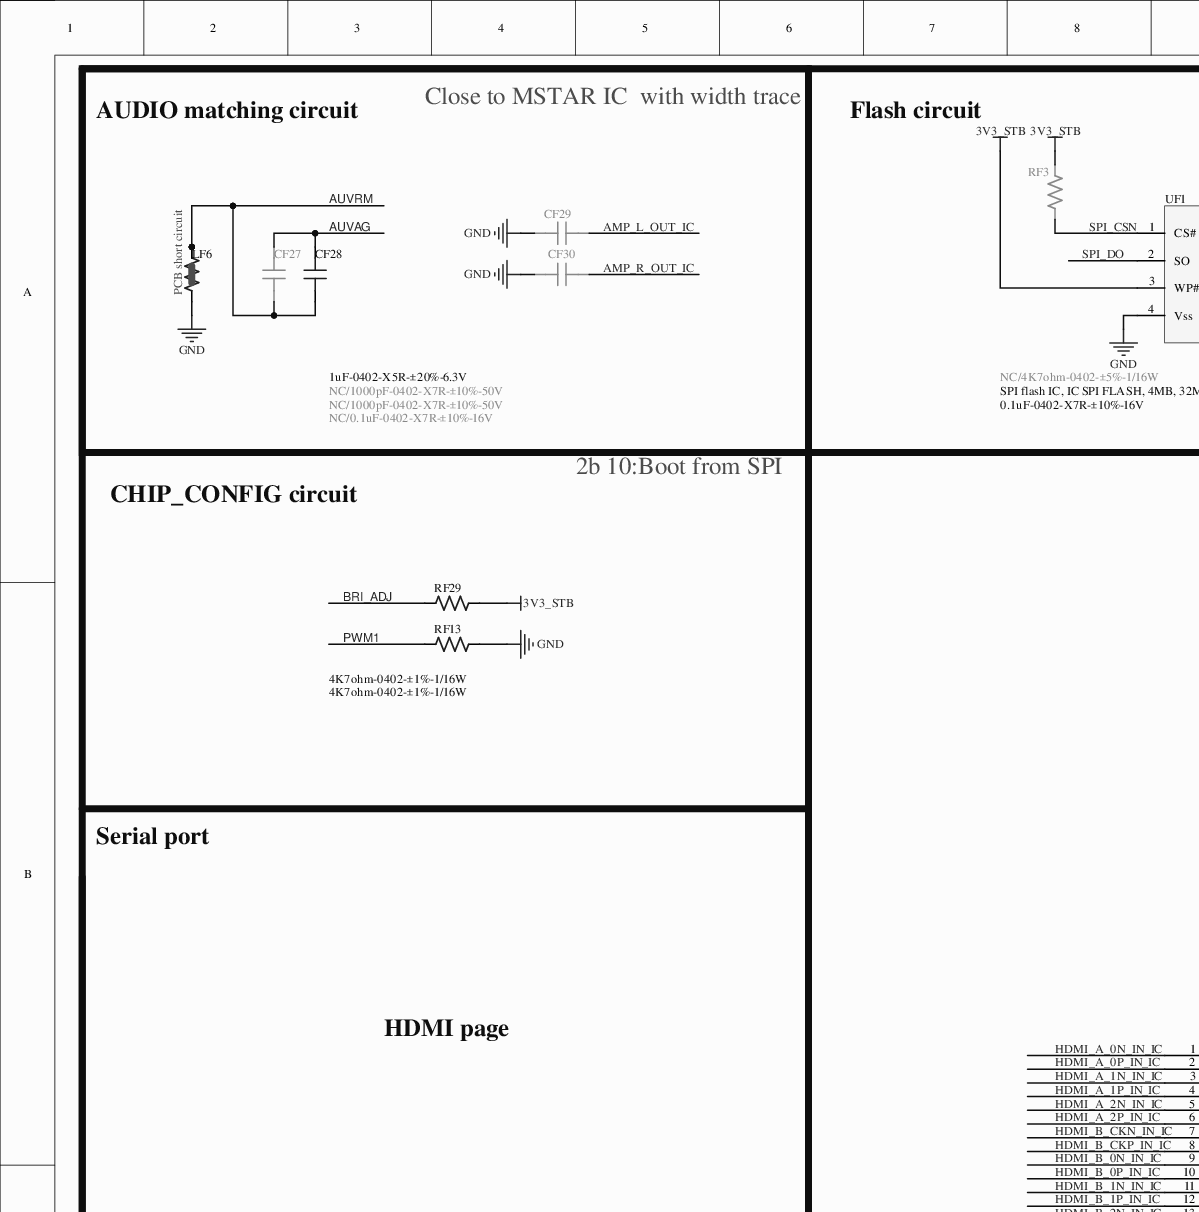
[diagram p0: MISC105950-36.SchDoc, top left]
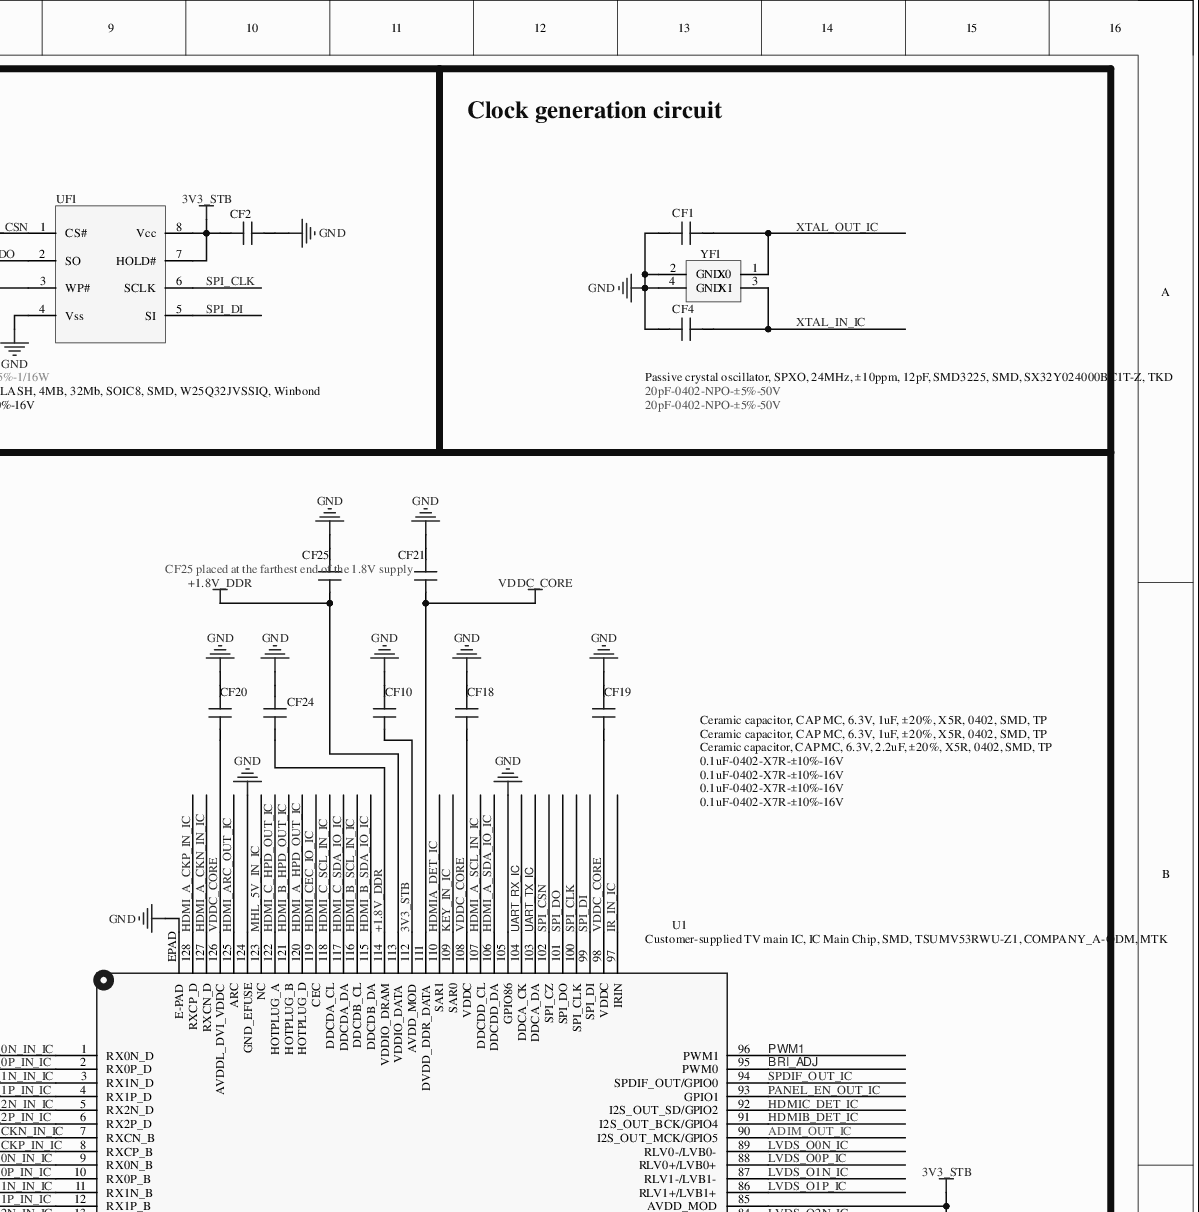
[diagram p1: MISC105950-36.SchDoc, top right]
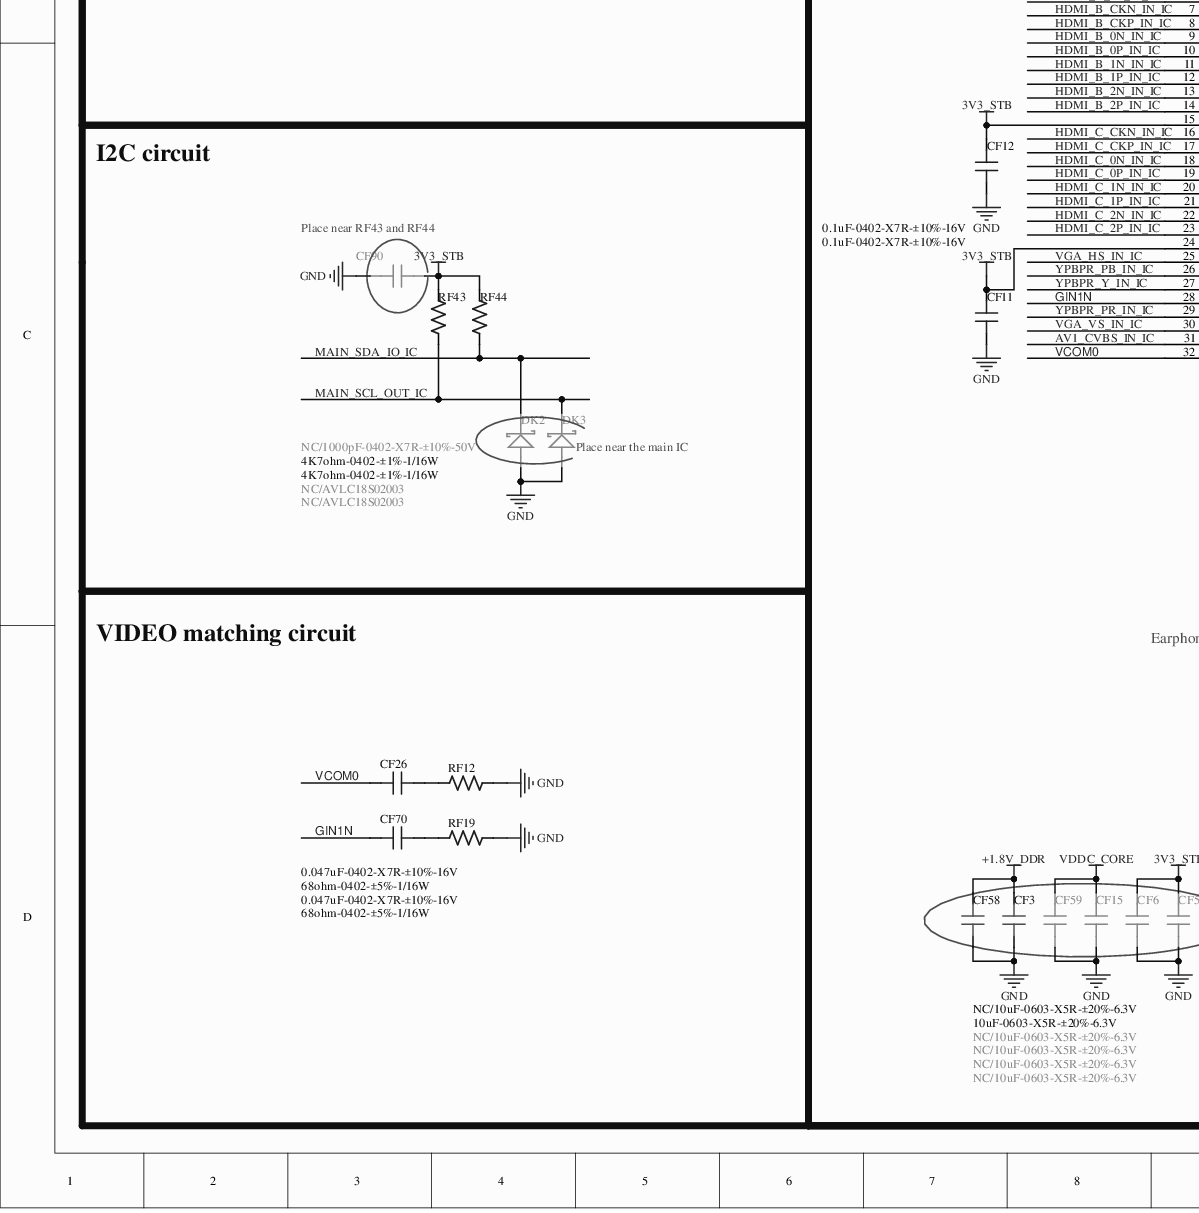
[diagram p2: MISC105950-36.SchDoc, bottom left]
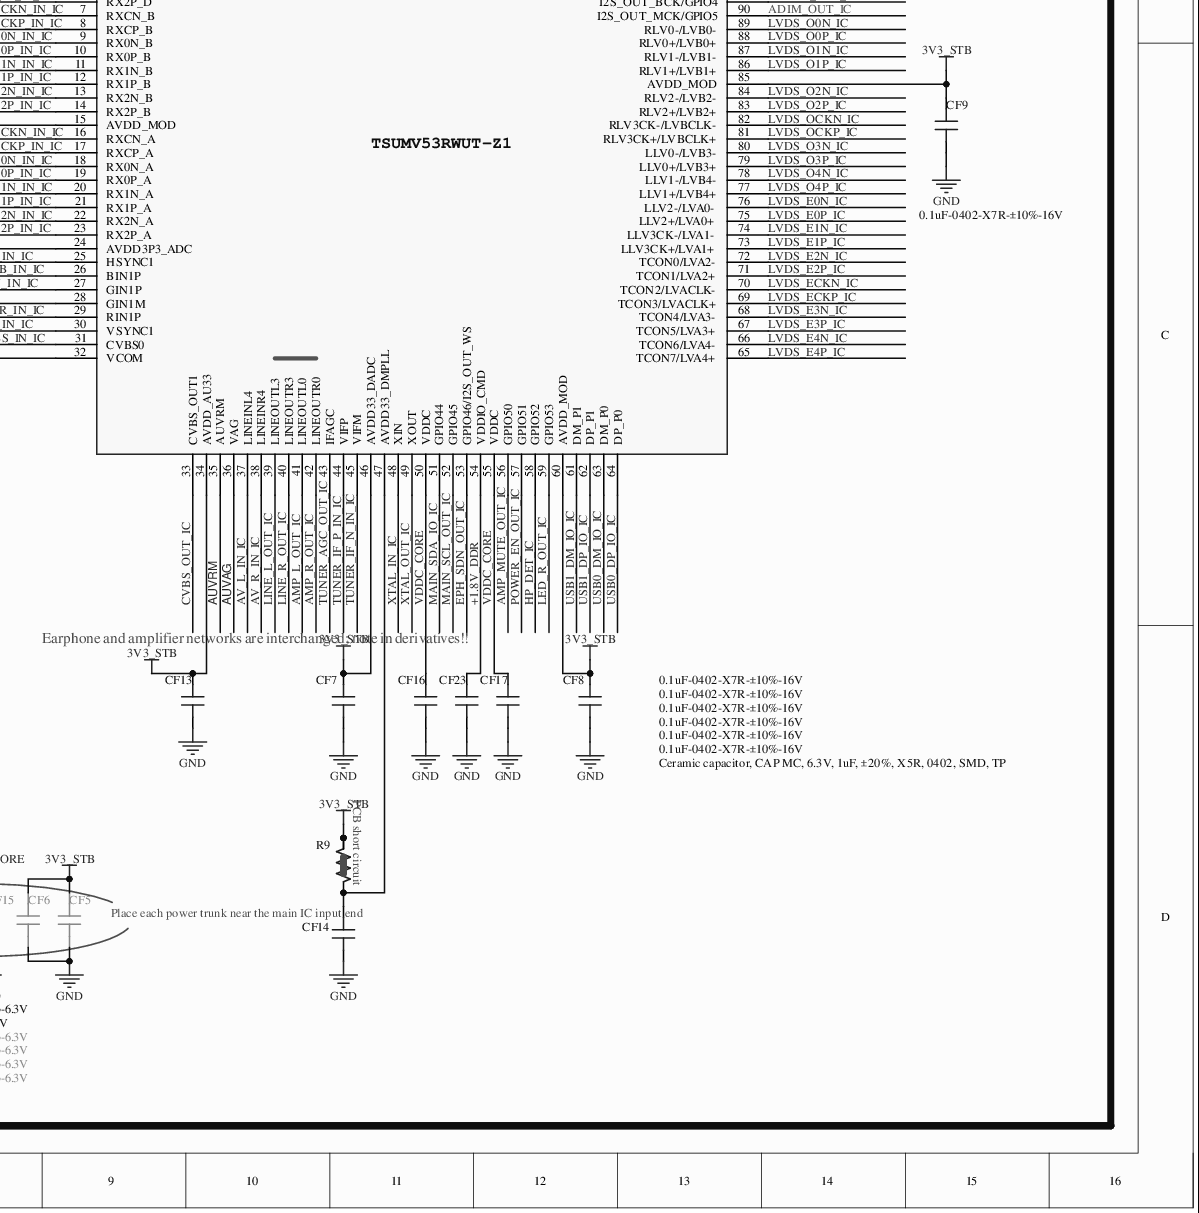
[diagram p3: MISC105950-36.SchDoc, bottom right]
# Altium project MISC105950-48.PrjPCB (part 4 of 8)

## Sheet MISC105950-36.SchDoc
size 426 x 431 mm

### Parts
CF1  20pF-0402-NPO-±5%-50V  [C0402]
CF2  0.1uF-0402-X7R-±10%-16V  [C0402]
CF3  10uF-0603-X5R-±20%-6.3V  [C0603]
CF4  20pF-0402-NPO-±5%-50V  [C0402]
CF5  NC/10uF-0603-X5R-±20%-6.3V  [C0603]
CF6  NC/10uF-0603-X5R-±20%-6.3V  [C0603]
CF7  0.1uF-0402-X7R-±10%-16V  [C0402]
CF8  0.1uF-0402-X7R-±10%-16V  [C0402]
CF9  0.1uF-0402-X7R-±10%-16V  [C0402]
CF10  0.1uF-0402-X7R-±10%-16V  [C0402]
CF11  0.1uF-0402-X7R-±10%-16V  [C0402]
CF12  0.1uF-0402-X7R-±10%-16V  [C0402]
CF13  0.1uF-0402-X7R-±10%-16V  [C0402]
CF14  0.1uF-0402-X7R-±10%-16V  [C0402]
CF15  NC/10uF-0603-X5R-±20%-6.3V  [C0603]
CF16  0.1uF-0402-X7R-±10%-16V  [C0402]
CF17  0.1uF-0402-X7R-±10%-16V  [C0402]
CF18  0.1uF-0402-X7R-±10%-16V  [C0402]
CF19  0.1uF-0402-X7R-±10%-16V  [C0402]
CF20  0.1uF-0402-X7R-±10%-16V  [C0402]
CF21  Ceramic capacitor, CAP MC, 6.3V, 1uF, ±20%, X5R, 0402, SMD, TP  [C0402]
CF23  Ceramic capacitor, CAP MC, 6.3V, 1uF, ±20%, X5R, 0402, SMD, TP  [C0402]
CF24  Ceramic capacitor, CAP MC, 6.3V, 1uF, ±20%, X5R, 0402, SMD, TP  [C0402]
CF25  Ceramic capacitor, CAP MC, 6.3V, 2.2uF, ±20%, X5R, 0402, SMD, TP  [C0402]
CF26  0.047uF-0402-X7R-±10%-16V  [C0402]
CF27  NC/0.1uF-0402-X7R-±10%-16V  [C0402]
CF28  1uF-0402-X5R-±20%-6.3V  [C0402]
CF29  NC/1000pF-0402-X7R-±10%-50V  [C0402]
CF30  NC/1000pF-0402-X7R-±10%-50V  [C0402]
CF58  NC/10uF-0603-X5R-±20%-6.3V  [C0603]
CF59  NC/10uF-0603-X5R-±20%-6.3V  [C0603]
CF70  0.047uF-0402-X7R-±10%-16V  [C0402]
CF90  NC/1000pF-0402-X7R-±10%-50V  [C0402]
DK2  NC/AVLC18S02003  [DIODE-S0402]
DK3  NC/AVLC18S02003  [DIODE-S0402]
LF6  NC/0ohm-0402-PCB  [R0402SC]  (value not drawn)
R9  NC/0ohm-0402-PCB  [R0402SC]  (value not drawn)
RF3  NC/4K7ohm-0402-±5%-1/16W  [R0402]
RF12  68ohm-0402-±5%-1/16W  [R0402]
RF13  4K7ohm-0402-±1%-1/16W  [R0402]
RF19  68ohm-0402-±5%-1/16W  [R0402]
RF29  4K7ohm-0402-±1%-1/16W  [R0402]
RF43  4K7ohm-0402-±1%-1/16W  [R0402]
RF44  4K7ohm-0402-±1%-1/16W  [R0402]
U1  Customer-supplied TV main IC, IC Main Chip, SMD, TSUMV53RWU-Z1, COMPANY_A-ODM, MTK  [QFN128/0.35-1]
UF1  SPI flash IC, IC SPI FLASH, 4MB, 32Mb, SOIC8, SMD, W25Q32JVSSIQ, Winbond  [SOIC8]
YF1  Passive crystal oscillator, SPXO, 24MHz, ±10ppm, 12pF, SMD3225, SMD, SX32Y024000BC1T-Z, TKD  [XTAL-S-3]

### Blocks framed on the sheet
Flash circuit: CF2 RF3 UF1
VIDEO matching circuit: CF26 CF70 RF12 RF19

### Nets
3V3_STB: CF2.2 CF5.2 CF6.2 CF7.2 CF8.2 CF9.2 CF10.2 CF11.1 CF12.2 CF13.2 CF90.1 R9.2 R9.3 RF3.2 RF29.2 RF43.1 RF44.1 U1.15(AVDD_MOD) U1.24(AVDD3P3_ADC) U1.34(AVDD_AU33) U1.46(AVDD33_DADC) U1.60(AVDD_MOD) U1.85(AVDD_MOD) U1.112(AVDD_MOD) UF1.3(WP#) UF1.7(HOLD#) UF1.8(Vcc)
+1.8V_DDR: CF3.2 CF23.2 CF24.2 CF25.1 CF58.2 U1.54(VDDIO_CMD) U1.113(VDDIO_DATA) U1.114(VDDIO_DRAM)
GND: CF1.1 CF2.1 CF3.1 CF4.1 CF5.1 CF6.1 CF7.1 CF8.1 CF9.1 CF10.1 CF11.2 CF12.1 CF13.1 CF14.1 CF15.1 CF16.1 CF17.1 CF18.2 CF19.2 CF20.1 CF21.2 CF23.1 CF24.1 CF25.2 CF29.2 CF30.2 CF58.1 CF59.1 CF90.2 DK2.A DK3.A LF6.1 RF12.2 RF13.2 RF19.2 U1.105(GPIO86) U1.124(GND_EFUSE) U1.EPAD(E-PAD) UF1.4(Vss) YF1.2(GND) YF1.4(GND)
VDDC_CORE: CF15.2 CF16.2 CF17.2 CF18.1 CF19.1 CF20.2 CF21.1 CF59.2 U1.50(VDDC) U1.55(VDDC) U1.98(VDDC) U1.108(VDDC) U1.111(DVDD_DDR_DATA) U1.126(AVDDL_DVI_VDDC)
ADIM_OUT_IC: U1.90(I2S_OUT_MCK/GPIO5)
AMP_L_OUT_IC: CF29.1 U1.41(LINEOUTL0)
AMP_MUTE_OUT_IC: U1.56(GPIO50)
AMP_R_OUT_IC: CF30.1 U1.42(LINEOUTR0)
AUVAG: CF27.2 CF28.2 U1.36(VAG)
AUVRM: CF27.1 CF28.1 LF6.2 LF6.3 U1.35(AUVRM)
AV1_CVBS_IN_IC: U1.31(CVBS0)
AV_L_IN_IC: U1.37(LINEINL4)
AV_R_IN_IC: U1.38(LINEINR4)
BRI_ADJ: RF29.1 U1.95(PWM0)
CVBS_OUT_IC: U1.33(CVBS_OUT1)
EPH_SDN_OUT_IC: U1.53(GPIO46/I2S_OUT_WS)
GIN1N: CF70.1 U1.28(GIN1M)
HDMI_A_0N_IN_IC: U1.1(RX0N_D)
HDMI_A_0P_IN_IC: U1.2(RX0P_D)
HDMI_A_1N_IN_IC: U1.3(RX1N_D)
HDMI_A_1P_IN_IC: U1.4(RX1P_D)
HDMI_A_2N_IN_IC: U1.5(RX2N_D)
HDMI_A_2P_IN_IC: U1.6(RX2P_D)
HDMI_A_CKN_IN_IC: U1.127(RXCN_D)
HDMI_A_CKP_IN_IC: U1.128(RXCP_D)
HDMI_A_HPD_OUT_IC: U1.120(HOTPLUG_D)
HDMI_A_SCL_IN_IC: U1.107(DDCDD_CL)
HDMI_A_SDA_IO_IC: U1.106(DDCDD_DA)
HDMI_ARC_OUT_IC: U1.125(ARC)
HDMI_B_0N_IN_IC: U1.9(RX0N_B)
HDMI_B_0P_IN_IC: U1.10(RX0P_B)
HDMI_B_1N_IN_IC: U1.11(RX1N_B)
HDMI_B_1P_IN_IC: U1.12(RX1P_B)
HDMI_B_2N_IN_IC: U1.13(RX2N_B)
HDMI_B_2P_IN_IC: U1.14(RX2P_B)
HDMI_B_CKN_IN_IC: U1.7(RXCN_B)
HDMI_B_CKP_IN_IC: U1.8(RXCP_B)
HDMI_B_HPD_OUT_IC: U1.121(HOTPLUG_B)
HDMI_B_SCL_IN_IC: U1.116(DDCDB_CL)
HDMI_B_SDA_IO_IC: U1.115(DDCDB_DA)
HDMI_C_0N_IN_IC: U1.18(RX0N_A)
HDMI_C_0P_IN_IC: U1.19(RX0P_A)
HDMI_C_1N_IN_IC: U1.20(RX1N_A)
HDMI_C_1P_IN_IC: U1.21(RX1P_A)
HDMI_C_2N_IN_IC: U1.22(RX2N_A)
HDMI_C_2P_IN_IC: U1.23(RX2P_A)
HDMI_C_CKN_IN_IC: U1.16(RXCN_A)
HDMI_C_CKP_IN_IC: U1.17(RXCP_A)
HDMI_C_HPD_OUT_IC: U1.122(HOTPLUG_A)
HDMI_C_SCL_IN_IC: U1.118(DDCDA_CL)
HDMI_C_SDA_IO_IC: U1.117(DDCDA_DA)
HDMI_CEC_IO_IC: U1.119(CEC)
HDMIA_DET_IC: U1.110(SAR1)
HDMIB_DET_IC: U1.91(I2S_OUT_BCK/GPIO4)
HDMIC_DET_IC: U1.92(I2S_OUT_SD/GPIO2)
HP_DET_IC: U1.58(GPIO52)
IR_IN_IC: U1.97(IRIN)
KEY_IN_IC: U1.109(SAR0)
LED_R_OUT_IC: U1.59(GPIO53)
LINE_L_OUT_IC: U1.39(LINEOUTL3)
LINE_R_OUT_IC: U1.40(LINEOUTR3)
LVDS_E0N_IC: U1.76(LLV2-/LVA0-)
LVDS_E0P_IC: U1.75(LLV2+/LVA0+)
LVDS_E1N_IC: U1.74(LLV3CK-/LVA1-)
LVDS_E1P_IC: U1.73(LLV3CK+/LVA1+)
LVDS_E2N_IC: U1.72(TCON0/LVA2-)
LVDS_E2P_IC: U1.71(TCON1/LVA2+)
LVDS_E3N_IC: U1.68(TCON4/LVA3-)
LVDS_E3P_IC: U1.67(TCON5/LVA3+)
LVDS_E4N_IC: U1.66(TCON6/LVA4-)
LVDS_E4P_IC: U1.65(TCON7/LVA4+)
LVDS_ECKN_IC: U1.70(TCON2/LVACLK-)
LVDS_ECKP_IC: U1.69(TCON3/LVACLK+)
LVDS_O0N_IC: U1.89(RLV0-/LVB0-)
LVDS_O0P_IC: U1.88(RLV0+/LVB0+)
LVDS_O1N_IC: U1.87(RLV1-/LVB1-)
LVDS_O1P_IC: U1.86(RLV1+/LVB1+)
LVDS_O2N_IC: U1.84(RLV2-/LVB2-)
LVDS_O2P_IC: U1.83(RLV2+/LVB2+)
LVDS_O3N_IC: U1.80(LLV0-/LVB3-)
LVDS_O3P_IC: U1.79(LLV0+/LVB3+)
LVDS_O4N_IC: U1.78(LLV1-/LVB4-)
LVDS_O4P_IC: U1.77(LLV1+/LVB4+)
LVDS_OCKN_IC: U1.82(RLV3CK-/LVBCLK-)
LVDS_OCKP_IC: U1.81(RLV3CK+/LVBCLK+)
MAIN_SCL_OUT_IC: DK3.K RF43.2 U1.52(GPIO45)
MAIN_SDA_IO_IC: DK2.K RF44.2 U1.51(GPIO44)
MHL_5V_IN_IC: U1.123(NC)
PANEL_EN_OUT_IC: U1.93(GPIO1)
POWER_EN_OUT_IC: U1.57(GPIO51)
PWM1: RF13.1 U1.96(PWM1)
SPDIF_OUT_IC: U1.94(SPDIF_OUT/GPIO0)
SPI_CLK: U1.100(SPI_CLK) UF1.6(SCLK)
SPI_CSN: RF3.1 U1.102(SPI_CZ) UF1.1(CS#)
SPI_DI: U1.99(SPI_DI) UF1.5(SI)
SPI_DO: U1.101(SPI_DO) UF1.2(SO)
TUNER_AGC_OUT_IC: U1.43(IFAGC)
TUNER_IF_N_IN_IC: U1.45(VIFM)
TUNER_IF_P_IN_IC: U1.44(VIFP)
UART_RX_IC: U1.104(DDCA_CK)
UART_TX_IC: U1.103(DDCA_DA)
USB0_DM_IO_IC: U1.63(DM_P0)
USB0_DP_IO_IC: U1.64(DP_P0)
USB1_DM_IO_IC: U1.61(DM_P1)
USB1_DP_IO_IC: U1.62(DP_P1)
VCOM0: CF26.1 U1.32(VCOM)
VGA_HS_IN_IC: U1.25(HSYNC1)
VGA_VS_IN_IC: U1.30(VSYNC1)
XTAL_IN_IC: CF4.2 U1.48(XIN) YF1.3(XI)
XTAL_OUT_IC: CF1.2 U1.49(XOUT) YF1.1(X0)
YPBPR_PB_IN_IC: U1.26(BIN1P)
YPBPR_PR_IN_IC: U1.29(RIN1P)
YPBPR_Y_IN_IC: U1.27(GIN1P)
NetCF14_2: CF14.2 R9.1 U1.47(AVDD33_DMPLL)
NetCF26_2: CF26.2 RF12.1
NetCF70_2: CF70.2 RF19.1

### Notes on the sheet
- AUDIO matching circuit
- Close to MSTAR IC  with width trace
- Clock generation circuit
- CHIP_CONFIG circuit
- 2b 10:Boot from SPI
- CF25 placed at the farthest end of the 1.8V supply
- Serial port
- HDMI page
- I2C circuit
- Place near RF43 and RF44
- (near DK3) Place near the main IC
- Earphone and amplifier networks are interchanged; note in derivatives!!
- (near CF14) Place each power trunk near the main IC input end

### Library data of the parts
CF1 CF4 = 30pF-0402-NPO-±5%-50V-D
CF2 CF7-CF10 CF12-CF14 CF17 CF27 = 0.1uF-0402-Y5V-+80%-20%-16V-D
CF3 CF5 CF6 CF15 CF58 CF59 = 004.003.0000383-D: Ceramic capacitor, CAP MC, 6.3V, 10uF, ±20%, X5R, 0603, SMD, TP-D
CF11 CF16 CF18-CF21 CF23-CF25 CF28 = 1uF-0402-X5R-±20%-6.3V-D
CF26 CF70 = 0.047uF-0402-X7R-±10%-16V-D
CF29 CF30 CF90 = 1000pF-0402-X7R-±10%-50V-D
DK2 DK3 = AVLC18S02003-D
LF6 R9 = 0ohm-0402-PCB-D
RF3 RF13 RF29 RF43 RF44 = 4K7ohm-0402-±5%-1/16W-D
RF12 RF19 = 68ohm-0402-±5%-1/16W-D
U1 = 004.016.0001146-D: TV main IC,IC Main Chip,TSUMV53RWUT-Z1,32bit,Single-Core,QFN128,SMD,Mstar-D
UF1 = SPI FLASH 芯片,IC SPI FLASH,32Mb,SOIC8,SMD,GD25Q32CSIG,GigaDevice-D
YF1 = 16.000MHz±20PPM-10PF-SMD3225-D: NC: GPS; PCB DECAL: TCXO_3225; Source_Path: EM_66_V2.0_201209181010.DSN; Value: 26M/0.5PPM/1.8V